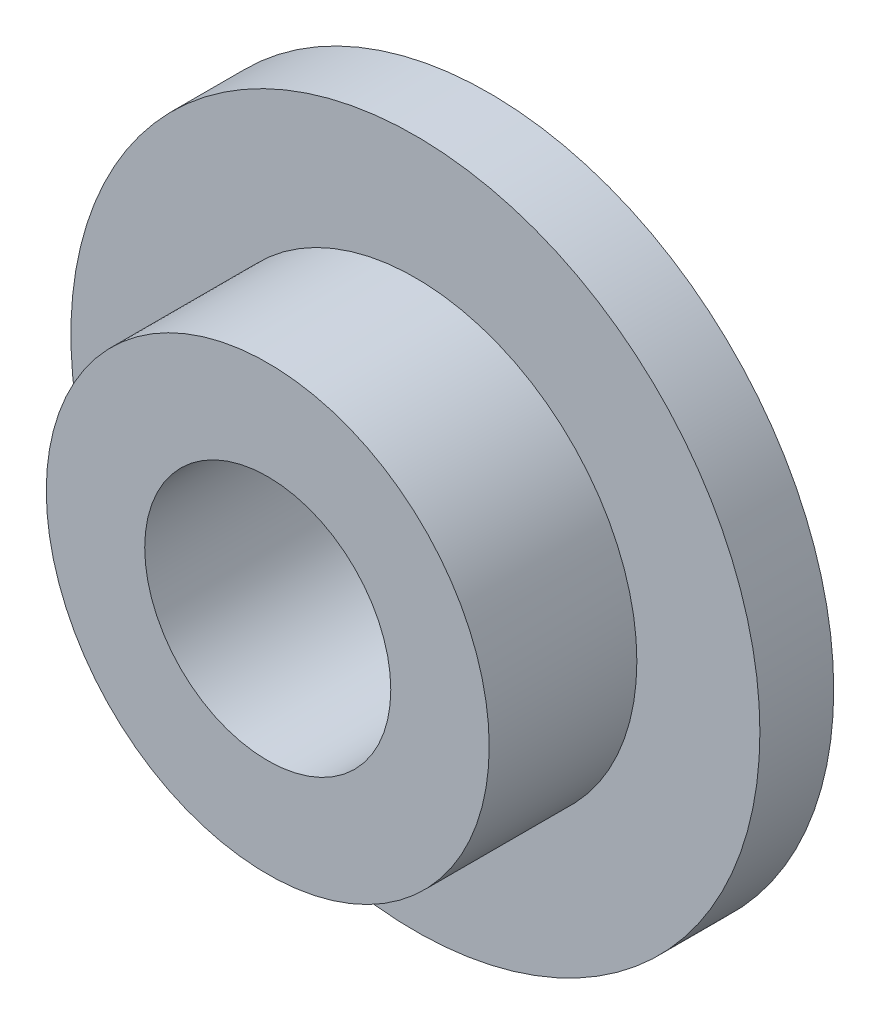
SolidWorks part; units mm, degrees
ref_plane "Front Plane" through (0, 0, 0) normal (0, 0, 1) x (1, 0, 0)
ref_plane "Top Plane" through (0, 0, 0) normal (0, 1, 0) x (1, 0, 0)
ref_plane "Right Plane" through (0, 0, 0) normal (1, 0, 0) x (0, 0, -1)
sketch "Sketch1" plane through (0, 0, 0) normal (0, 0, 1) x (1, 0, 0)
  circle A0 centre (0, 0) radius 14
  dimension "D1" = 28
extrude "Boss-Extrude1" add sketch "Sketch1" along normal blind 3
sketch "Sketch2" plane through (0, 0, 3) normal (0, 0, 1) x (1, 0, 0)
  circle A0 centre (0, 0) radius 9
  dimension "D1" = 18
extrude "Boss-Extrude2" add sketch "Sketch2" along normal blind 6
sketch "Sketch3" plane through (0, 0, 9) normal (0, 0, 1) x (1, 0, 0)
  circle A0 centre (0, 0) radius 5
  dimension "D1" = 10
extrude "Cut-Extrude1" cut sketch "Sketch3" against normal blind 12
